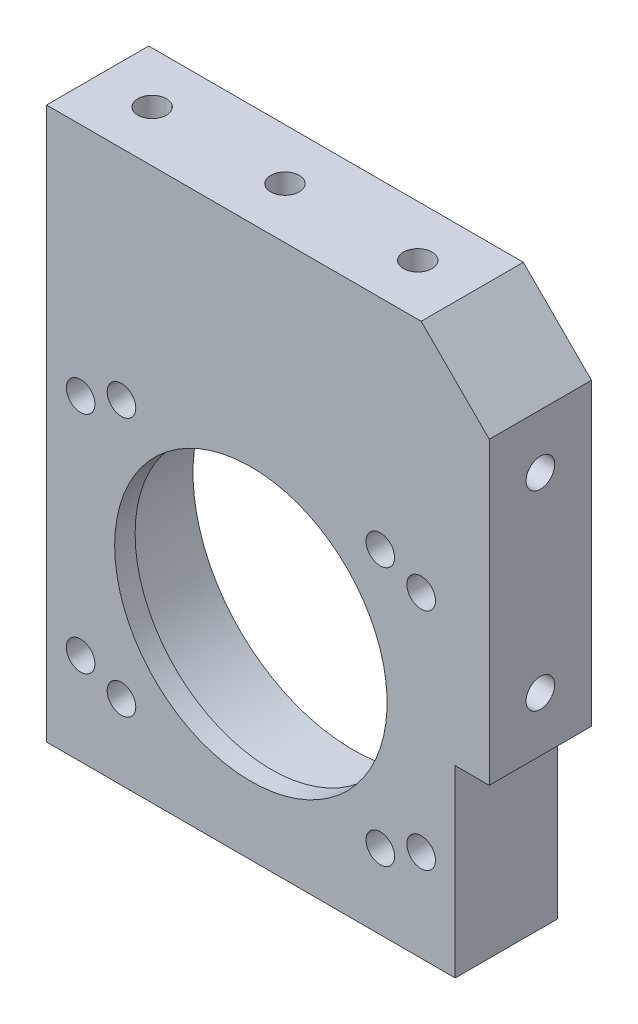
SolidWorks part; units mm, degrees
material "6061Al"
ref_plane "前视基准面" through (0, 0, 0) normal (0, 0, 1) x (1, 0, 0)
ref_plane "上视基准面" through (0, 0, 0) normal (0, 1, 0) x (1, 0, 0)
ref_plane "右视基准面" through (0, 0, 0) normal (1, 0, 0) x (0, 0, -1)
sketch "草图1" plane through (0, 0, 0) normal (0, 0, 1) x (1, 0, 0)
  line L1 (-32.5, -41) -> (32.5, -41)
  line L2 (-32.5, -41) -> (-32.5, 41)
  line L3 (-32.5, 41) -> (32.5, 41)
  line L4 (32.5, -41) -> (32.5, 41)
  line L5 (-32.5, -41) -> (32.5, 41) construction
  line L6 (-32.5, 41) -> (32.5, -41) construction
  point P0 (0, 0)
  dimension "D1" = 65
  dimension "D2" = 82
extrude "凸台-拉伸1" add sketch "草图1" along normal mid plane 15
sketch "草图10" plane through (0, 0, -7.5) normal (0, 0, 1) x (1, 0, 0)
  line L1 (-32.5, 41) -> (-32.5, -41) construction
  line L2 (-32.5, -41) -> (32.5, -41) construction
  circle A0 centre (-2.5, -11) radius 23.5
  dimension "D1" = 47
  dimension "D2" = 30
  dimension "D3" = 30
extrude "切除-拉伸1" cut sketch "草图10" along normal blind 12
sketch "草图12" plane through (0, 0, 4.5) normal (0, 0, -1) x (-1, 0, 0)
  circle A0 centre (2.5, -11) radius 20
  dimension "D1" = 40
extrude "切除-拉伸2" cut sketch "草图12" against normal through all
sketch "草图13" plane through (0, 0, 7.5) normal (0, 0, 1) x (1, 0, 0)
  line L0 (-32.5, -41) -> (32.5, -41) construction
  line L1 (27.5, -41) -> (32.5, -41)
  line L2 (27.5, -41) -> (27.5, -14)
  line L3 (27.5, -14) -> (32.5, -14)
  line L4 (32.5, -41) -> (32.5, -14)
  line L5 (32.5, -41) -> (32.5, 41) construction
  line L6 (-32.5, 41) -> (-32.5, -41) construction
  line L7 (32.5, 41) -> (-32.5, 41) construction
  dimension "D1" = 60
  dimension "D2" = 55
extrude "切除-拉伸3" cut sketch "草图13" against normal through all
fillet "圆角1" [suppressed] radius 5
hole_wizard "M5 螺纹孔1" positions "草图14" profile "草图15" tap size "M5" standard "ISO" end condition through all
sketch "草图14" plane through (0, 0, -7.5) normal (0, 0, -1) x (-1, 0, 0)
  circle A0 centre (2.5, -11) radius 20 construction
  point P13 (-22.5, 5.5)
  point P16 (-22.5, -27.5)
  point P19 (27.5, -27.5)
  point P22 (27.5, 5.5)
  dimension "D1" = 25
  dimension "D2" = 25
  dimension "D3" = 16.5
  dimension "D4" = 16.5
sketch "草图15" plane through (22.5, 5.5, -7.5) normal (1, 0, 0) x (0, 1, 0)
  line L0 (0, 0) -> (0, 15)
  line L1 (0, 15) -> (2.1, 15)
  line L2 (2.1, 15) -> (2.1, 0)
  line L5 (2.1, 0) -> (0, 0)
  line L11 (0, -6.35) -> (0, 107.95) construction
  dimension "通孔螺纹孔钻头直径" = 4.2
  dimension "通孔螺纹孔钻头深度" = 15
cosmetic thread "孔螺蚊线1" parameters "D2"=5
cosmetic thread "孔螺蚊线2" parameters "D2"=5
cosmetic thread "孔螺蚊线3" parameters "D2"=5
cosmetic thread "孔螺蚊线4" parameters "D2"=5
hole_wizard "M5 螺纹孔2" positions "草图16" profile "草图17" tap size "M5" standard "ISO" end condition through all
sketch "草图16" plane through (0, 0, 7.5) normal (0, 0, 1) x (1, 0, 0)
  circle A0 centre (-2.5, -11) radius 20 construction
  point P0 (-21.5, 8)
  point P3 (-21.5, -30)
  point P6 (16.5, -30)
  point P9 (16.5, 8)
sketch "草图17" plane through (-21.5, 8, 7.5) normal (1, 0, 0) x (0, -1, 0)
  line L0 (0, 0) -> (0, 15)
  line L1 (0, 15) -> (2.1, 15)
  line L2 (2.1, 15) -> (2.1, 0)
  line L5 (2.1, 0) -> (0, 0)
  line L11 (0, -6.35) -> (0, 107.95) construction
  dimension "通孔螺纹孔钻头直径" = 4.2
  dimension "通孔螺纹孔钻头深度" = 15
cosmetic thread "孔螺蚊线5" parameters "D2"=5
cosmetic thread "孔螺蚊线6" parameters "D2"=5
cosmetic thread "孔螺蚊线7" parameters "D2"=5
cosmetic thread "孔螺蚊线8" parameters "D2"=5
other "移动面1" face at (0, 41, 0) parameters "D1"=1
other "移动面2" [suppressed] parameters "D1"=8
hole_wizard "M5 螺纹孔4" positions "草图20" profile "草图21" tap size "M5" standard "ISO"
sketch "草图20" plane through (32.5, 0, 0) normal (1, 0, 0) x (0, 0, -1)
  line L4 (-7.5, 40) -> (7.5, 40) construction
  point P0 (0, -6)
  point P3 (0, 22)
  dimension "D1" = 28
  dimension "D2" = 18
sketch "草图21" plane through (32.5, -6, 0) normal (0, 1, 0) x (0, 0, -1)
  line L0 (0, 0) -> (0, 13.6618)
  line L1 (0, 13.6618) -> (2.1, 12.4)
  line L2 (2.1, 12.4) -> (2.1, 0)
  line L5 (2.1, 0) -> (0, 0)
  line L10 (0, 13.6618) -> (-2.1, 12.4) construction
  line L11 (0, -6.35) -> (0, 107.95) construction
  dimension "螺纹孔钻头直径" = 4.2
  dimension "螺纹孔钻头深度" = 12.4
  dimension "导头角度" = 118
cosmetic thread "孔螺蚊线12" parameters "D1"=10, "D2"=5
cosmetic thread "孔螺蚊线13" parameters "D1"=10, "D2"=5
chamfer "倒角2" distance 10 angle 45 1 edges at (32.5, 40, 0)
hole_wizard "M5 螺纹孔3" positions "草图18" profile "草图19" tap size "M5" standard "ISO"
sketch "草图18" plane through (0, 40, 0) normal (0, 1, 0) x (1, 0, 0)
  line L0 (-5, 7.5) -> (-5, -7.5) construction
  line L1 (22.5, 7.5) -> (-32.5, 7.5) construction
  line L2 (22.5, -7.5) -> (-32.5, -7.5) construction
  line L4 (-32.5, -7.5) -> (-32.5, 7.5) construction
  point P12 (-24.5, 0)
  point P25 (-5, 0)
  point P27 (14.5, 0)
  dimension "D1" = 8
sketch "草图19" plane through (-24.5, 40, 0) normal (1, 0, 0) x (0, 0, 1)
  line L0 (0, 0) -> (0, 13.6618)
  line L1 (0, 13.6618) -> (2.1, 12.4)
  line L2 (2.1, 12.4) -> (2.1, 0)
  line L5 (2.1, 0) -> (0, 0)
  line L10 (0, 13.6618) -> (-2.1, 12.4) construction
  line L11 (0, -6.35) -> (0, 107.95) construction
  dimension "螺纹孔钻头直径" = 4.2
  dimension "螺纹孔钻头深度" = 12.4
  dimension "导头角度" = 118
cosmetic thread "孔螺蚊线9" parameters "D1"=10, "D2"=5
cosmetic thread "孔螺蚊线10" parameters "D1"=10, "D2"=5
cosmetic thread "孔螺蚊线14" parameters "D1"=10, "D2"=5
move or copy body "实体-移动/复制1" [suppressed] bodies to move or copy 114 parameters "D1"=0, "D2"=0, "D3"=0
equation "\"D1@草图16\"=\"D2@草图16\""
